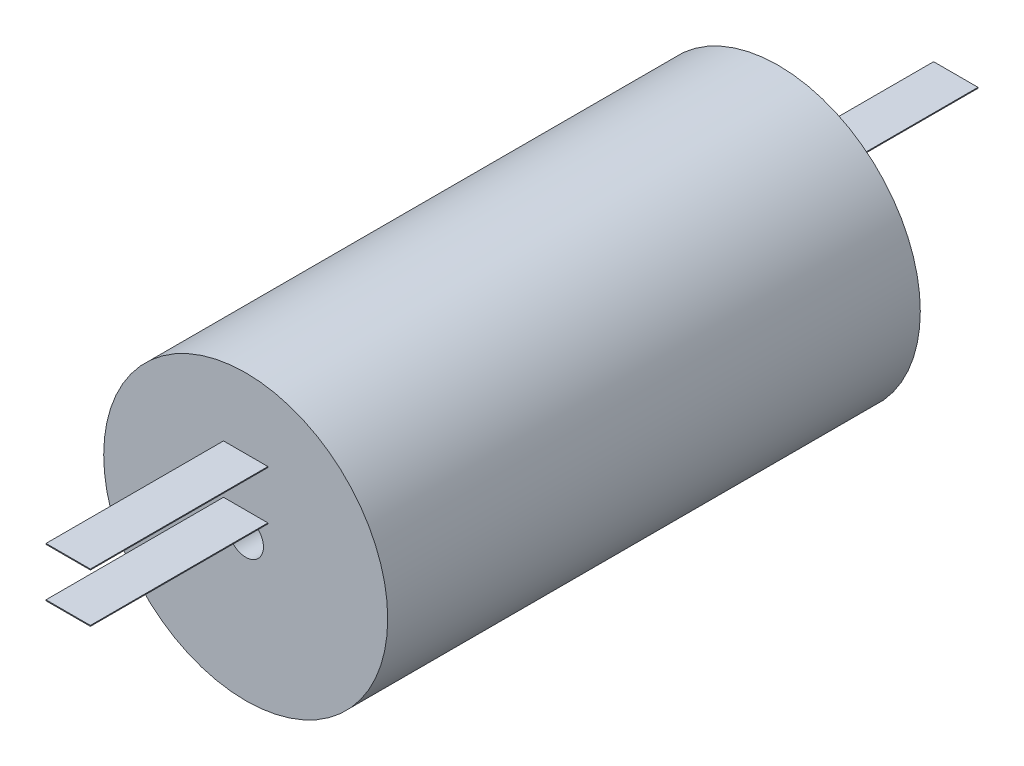
SolidWorks part; units mm, degrees
material "6061"
ref_plane "Front Plane" through (0, 0, 0) normal (0, 0, 1) x (1, 0, 0)
ref_plane "Top Plane" through (0, 0, 0) normal (0, 1, 0) x (1, 0, 0)
ref_plane "Right Plane" through (0, 0, 0) normal (1, 0, 0) x (0, 0, -1)
sketch "Sketch1" plane through (0, 0, 0) normal (0, 0, 1) x (1, 0, 0)
  circle A0 centre (0, 0) radius 16
  circle A1 centre (0, 0) radius 2
  dimension "D1" = 4
  dimension "D2" = 32
extrude "Boss-Extrude1" add sketch "Sketch1" along normal blind 60
sketch "Sketch2" plane through (0, 0, 0) normal (0, 0, -1) x (-1, 0, 0)
  line L0 (0, 0) -> (0, 16) construction
  line L2 (-2.5, 5.1) -> (2.5, 5.1)
  line L3 (-2.5, 5.1) -> (-2.5, 5)
  line L4 (-2.5, 5) -> (2.5, 5)
  line L5 (2.5, 5.1) -> (2.5, 5)
  line L6 (-2.5, 5.1) -> (2.5, 5) construction
  line L7 (-2.5, 5) -> (2.5, 5.1) construction
  circle A0 centre (0, 0) radius 16 construction
  point P6 (0, 5.05)
  dimension "D1" = 5
  dimension "D2" = 0.1
  dimension "D3" = 5
extrude "Boss-Extrude2" add sketch "Sketch2" along normal blind 20
sketch "Sketch3" plane through (0, 0, 60) normal (0, 0, 1) x (1, 0, 0)
  line L0 (0, 0) -> (0, 16) construction
  line L2 (-2.5, 8.1) -> (2.5, 8.1)
  line L3 (-2.5, 8.1) -> (-2.5, 8)
  line L4 (-2.5, 8) -> (2.5, 8)
  line L5 (2.5, 8.1) -> (2.5, 8)
  line L6 (-2.5, 8.1) -> (2.5, 8) construction
  line L7 (-2.5, 8) -> (2.5, 8.1) construction
  line L8 (-2.5, 2.6) -> (2.5, 2.6)
  line L9 (-2.5, 2.6) -> (-2.5, 2.5)
  line L10 (-2.5, 2.5) -> (2.5, 2.5)
  line L11 (2.5, 2.6) -> (2.5, 2.5)
  circle A0 centre (0, 0) radius 16 construction
  point P6 (0, 8.05)
  dimension "D1" = 0.1
  dimension "D2" = 5
  dimension "D3" = 8
  dimension "D4" = 2.5
extrude "Boss-Extrude3" add sketch "Sketch3" along normal blind 20
